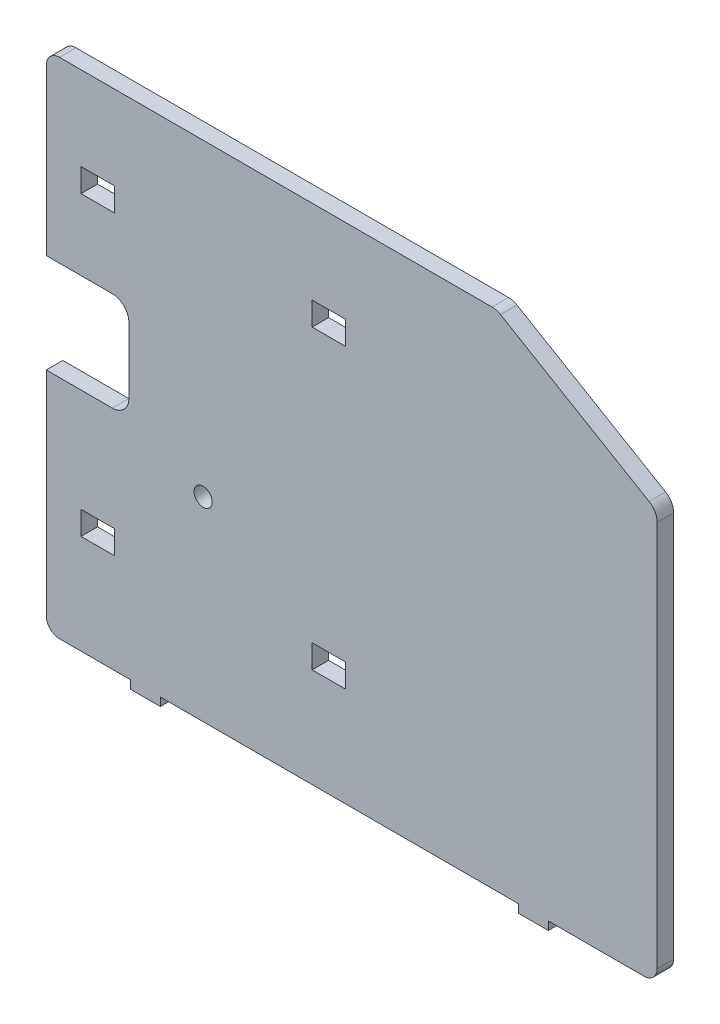
SolidWorks part; units mm, degrees
material "Q235"
ref_plane "Front Plane" through (0, 0, 0) normal (0, 0, 1) x (1, 0, 0)
ref_plane "Top Plane" through (0, 0, 0) normal (0, 1, 0) x (1, 0, 0)
ref_plane "Right Plane" through (0, 0, 0) normal (1, 0, 0) x (0, 0, -1)
sketch "Sketch1" plane through (0, 0, 0) normal (0, 0, 1) x (1, 0, 0)
  line L0 (538.1081, 869.5394) -> (628.1081, 816.5185)
  line L1 (633.0022, 807.9202) -> (633.0022, 573.9411)
  line L2 (533.0022, 870.9411) -> (271.0022, 870.9411)
  line L3 (284.0022, 626.1411) -> (284.0022, 640.3411)
  line L4 (284.0022, 640.3411) -> (304.2022, 640.3411)
  line L5 (304.2022, 640.3411) -> (304.2022, 626.1411)
  line L6 (304.2022, 626.1411) -> (284.0022, 626.1411)
  line L7 (424.0022, 626.1411) -> (424.0022, 640.3411)
  line L8 (424.0022, 640.3411) -> (444.2022, 640.3411)
  line L9 (444.2022, 640.3411) -> (444.2022, 626.1411)
  line L10 (444.2022, 626.1411) -> (424.0022, 626.1411)
  line L11 (284.0022, 805.9411) -> (284.0022, 820.1411)
  line L12 (284.0022, 820.1411) -> (304.2022, 820.1411)
  line L13 (304.2022, 820.1411) -> (304.2022, 805.9411)
  line L14 (304.2022, 805.9411) -> (284.0022, 805.9411)
  line L15 (424.0022, 805.9411) -> (424.0022, 820.1411)
  line L16 (424.0022, 820.1411) -> (444.2022, 820.1411)
  line L17 (444.2022, 820.1411) -> (444.2022, 805.9411)
  line L18 (444.2022, 805.9411) -> (424.0022, 805.9411)
  line L19 (263.0022, 862.9411) -> (263.0022, 762.9411)
  line L20 (263.0022, 762.9411) -> (303.0022, 762.9411)
  line L21 (313.0022, 752.9411) -> (313.0022, 712.9411)
  line L22 (303.0022, 702.9411) -> (263.0022, 702.9411)
  line L23 (263.0022, 702.9411) -> (263.0022, 573.9411)
  line L24 (314.0611, 565.9411) -> (314.0611, 560.9411)
  line L25 (314.0611, 560.9411) -> (332.0611, 560.9411)
  line L26 (332.0611, 560.9411) -> (332.0611, 565.9411)
  line L27 (549.0611, 565.9411) -> (549.0611, 560.9411)
  line L28 (549.0611, 560.9411) -> (567.0611, 560.9411)
  line L29 (567.0611, 560.9411) -> (567.0611, 565.9411)
  line L30 (271.0022, 565.9411) -> (314.0611, 565.9411)
  line L31 (332.0611, 565.9411) -> (549.0611, 565.9411)
  line L32 (567.0611, 565.9411) -> (625.0022, 565.9411)
  arc A0 (633.0022, 807.9202) -> (628.1081, 816.5185) centre (623.0022, 807.9202) ccw
  arc A1 (538.1081, 869.5394) -> (533.0022, 870.9411) centre (533.0022, 860.9411) ccw
  arc A2 (263.0022, 573.9411) -> (271.0022, 565.9411) centre (271.0022, 573.9411) ccw
  arc A3 (625.0022, 565.9411) -> (633.0022, 573.9411) centre (625.0022, 573.9411) ccw
  arc A4 (271.0022, 870.9411) -> (263.0022, 862.9411) centre (271.0022, 862.9411) ccw
  arc A5 (313.0022, 752.9411) -> (303.0022, 762.9411) centre (303.0022, 752.9411) ccw
  arc A6 (303.0022, 702.9411) -> (313.0022, 712.9411) centre (303.0022, 712.9411) ccw
  circle A7 centre (358.0022, 683.9411) radius 5.5
extrude "Boss-Extrude1" add sketch "Sketch1" along normal blind 10
equation "\"图号代码1\"= \"图号代码\""
equation "\"名称代码2\"= \"名称代码\""
